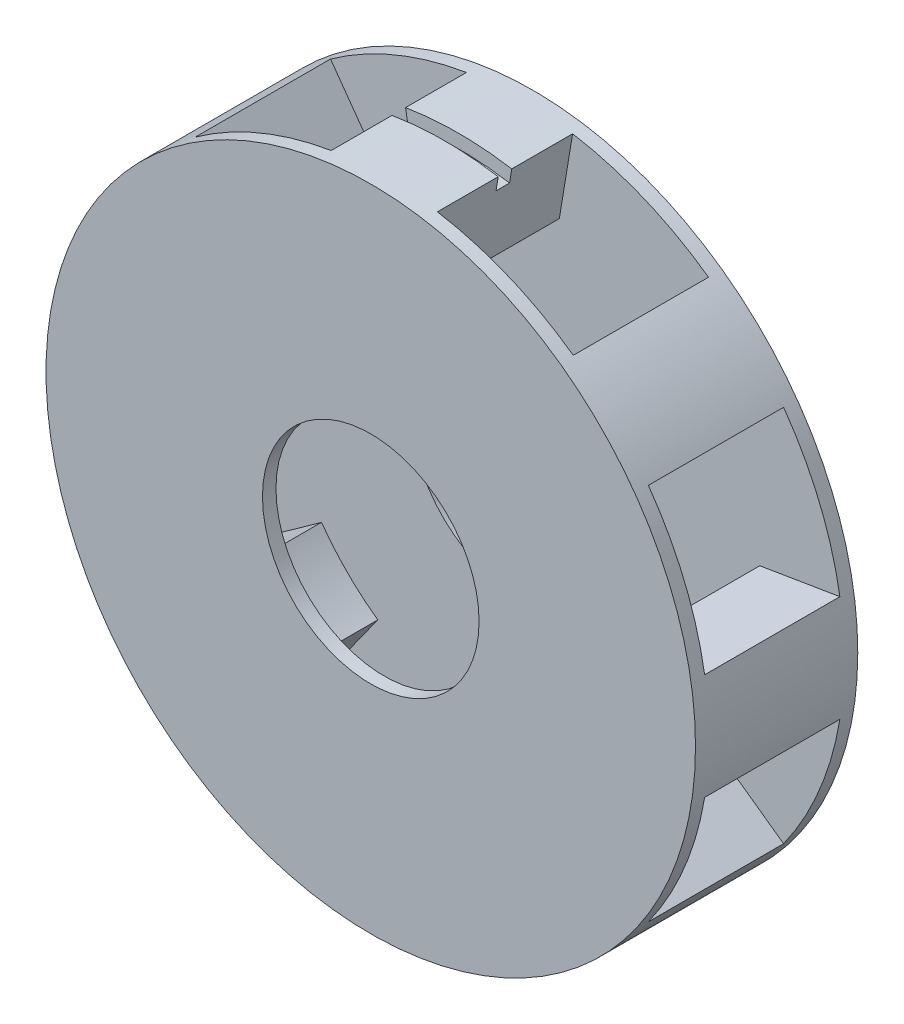
SolidWorks part; units mm, degrees
ref_plane "Front Plane" through (0, 0, 0) normal (0, 0, 1) x (1, 0, 0)
ref_plane "Top Plane" through (0, 0, 0) normal (0, 1, 0) x (1, 0, 0)
ref_plane "Right Plane" through (0, 0, 0) normal (1, 0, 0) x (0, 0, -1)
sketch "Sketch1" plane through (0, 0, 0) normal (0, 0, 1) x (1, 0, 0)
  circle A0 centre (0, 0) radius 120
  circle A1 centre (0, 0) radius 150
  dimension "D1" = 240
  dimension "D2" = 300
extrude "Boss-Extrude1" add sketch "Sketch1" along normal blind 59.97
sketch "Sketch2" plane through (0, 0, 59.97) normal (0, 0, 1) x (1, 0, 0)
  circle A0 centre (0, 0) radius 90
  circle A1 centre (0, 0) radius 120
  dimension "D1" = 180
extrude "Boss-Extrude2" add sketch "Sketch2" against normal blind 59.97
sketch "Sketch3" plane through (0, 0, 59.97) normal (0, 0, 1) x (1, 0, 0)
  line L1 (-15.6631, 118.9734) -> (-19.5789, 148.7167)
  line L2 (15.6631, 118.9734) -> (19.5789, 148.7167)
  circle A0 centre (0, 0) radius 150 construction
  arc A1 (15.6631, 118.9734) -> (-15.6631, 118.9734) centre (0, 0) ccw
  arc A2 (-19.5789, 148.7167) -> (19.5789, 148.7167) centre (0, 0) cw
  dimension "D2" = 120
extrude "Cut-Extrude1" cut sketch "Sketch3" against normal blind 59.97
pattern_circular "CirPattern1" count 8 over 360 about axis through (0, 0, 0) along (0, 0, 1) of "Cut-Extrude1"
ref_plane "Plane1" through (0, 0, 54.97) normal (0, 0, 1) x (1, 0, 0)
sketch "Sketch5" plane through (0, 0, 54.97) normal (0, 0, 1) x (1, 0, 0)
  line L1 (14.7146, 88.789) -> (24.5244, 147.9816)
  line L4 (52.3785, 73.1881) -> (87.2975, 121.9801)
  arc A0 (91.3142, 119.003) -> (19.5789, 148.7167) centre (0, 0) ccw construction
  arc A1 (14.7146, 88.789) -> (52.3785, 73.1881) centre (0, 0) cw
  circle A2 centre (0, 0) radius 90 construction
  arc A3 (24.5244, 147.9816) -> (87.2975, 121.9801) centre (0, 0) cw
extrude "Cut-Extrude2" cut sketch "Sketch5" against normal blind 49.97
pattern_circular "CirPattern2" count 8 over 360 about axis through (0, 0, 0) along (0, 0, 1) of "Cut-Extrude2"
sketch "Sketch6" plane through (0, 0, 59.97) normal (0, 0, 1) x (1, 0, 0)
  circle A0 centre (0, 0) radius 90
  circle A1 centre (0, 0) radius 40.03
  dimension "D1" = 80.06
extrude "Boss-Extrude3" add sketch "Sketch6" against normal blind 5
sketch "Sketch7" plane through (0, 0, 0) normal (0, 0, -1) x (-1, 0, 0)
  circle A0 centre (0, 0) radius 90
  circle A1 centre (0, 0) radius 40.03
extrude "Boss-Extrude4" add sketch "Sketch7" against normal blind 5
sketch "Sketch8" plane through (0, 0, 0) normal (0, 0, -1) x (-1, 0, 0)
  circle A0 centre (0, 0) radius 150
  circle A1 centre (0, 0) radius 120
extrude "Cut-Extrude3" cut sketch "Sketch8" against normal blind 80
sketch "Sketch10" plane through (0, 0, 0) normal (0.9865, -0.1635, 0) x (0, 0, -1)
  line L2 (-32.485, 120) -> (-32.485, 115)
  line L3 (-32.485, 120) -> (-27.485, 120)
  line L5 (-32.485, 115) -> (-27.485, 115)
  line L6 (-27.485, 120) -> (-27.485, 115)
  dimension "D2" = 5
sketch "Sketch11" plane through (0, 0, 0) normal (0, 1, 0) x (1, 0, 0)
  line L0 (0, 0) -> (0, -59.97)
  line L1 (-120, -59.97) -> (120, -59.97) construction
revolve "Cut-Revolve1" cut sketch "Sketch10" angle 30 about L0
